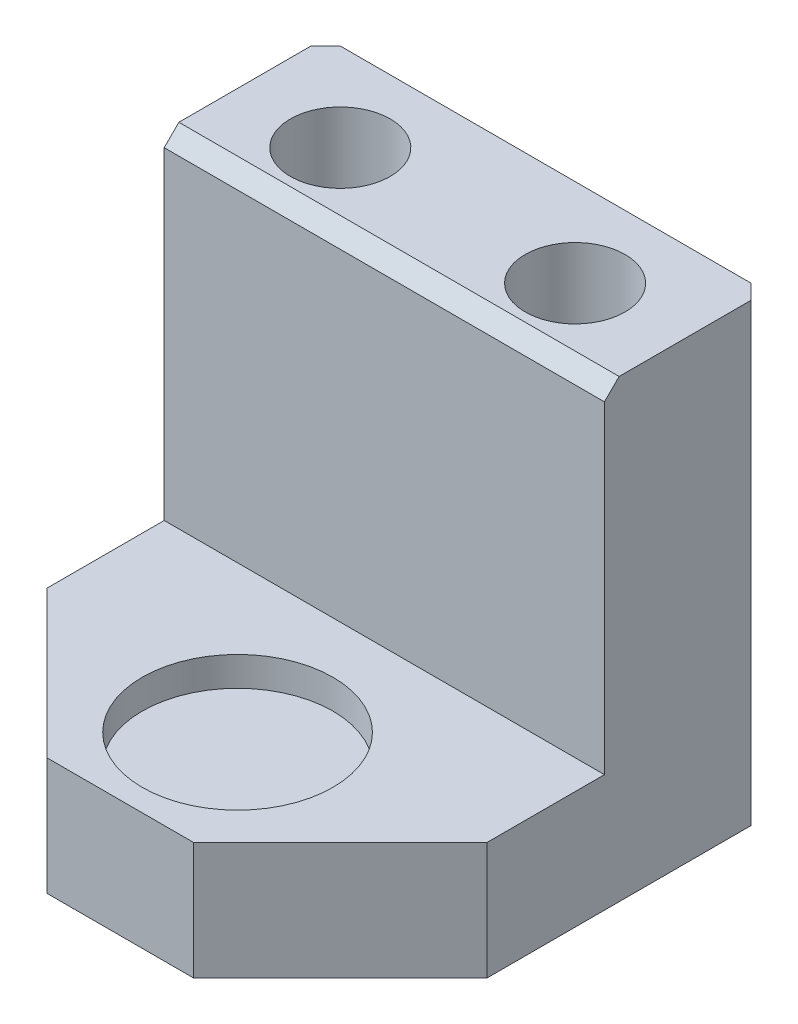
SolidWorks part; units mm, degrees
ref_plane "Front Plane" through (0, 0, 0) normal (0, 0, 1) x (1, 0, 0)
ref_plane "Top Plane" through (0, 0, 0) normal (0, 1, 0) x (1, 0, 0)
ref_plane "Right Plane" through (0, 0, 0) normal (1, 0, 0) x (0, 0, -1)
sketch "Sketch1" plane through (0, 0, 0) normal (0, 0, 1) x (1, 0, 0)
  line L1 (-7.5, -7.75) -> (7.5, -7.75)
  line L2 (-7.5, -7.75) -> (-7.5, 7.75)
  line L3 (-7.5, 7.75) -> (7.5, 7.75)
  line L4 (7.5, -7.75) -> (7.5, 7.75)
  line L5 (-7.5, -7.75) -> (7.5, 7.75) construction
  line L6 (-7.5, 7.75) -> (7.5, -7.75) construction
  point P0 (0, 0)
  dimension "D1" = 15
  dimension "D2" = 15.5
extrude "Boss-Extrude1" add sketch "Sketch1" along normal blind 6
sketch "Sketch2" plane through (0, 0, 6) normal (0, 0, 1) x (1, 0, 0)
  line L0 (7.5, -7.75) -> (7.5, 7.75) construction
  line L1 (-7.5, -7.75) -> (7.5, -7.75)
  line L2 (-7.5, -7.75) -> (-7.5, -3.75)
  line L3 (-7.5, -3.75) -> (7.5, -3.75)
  line L4 (7.5, -7.75) -> (7.5, -3.75)
  dimension "D1" = 4
extrude "Boss-Extrude2" add sketch "Sketch2" along normal blind 9
sketch "Sketch3" plane through (0, -3.75, 0) normal (0, 1, 0) x (1, 0, 0)
  line L0 (0, 0) -> (0, -20.2651) construction
  circle A0 centre (0, -11) radius 3.25
  dimension "D2" = 6.5
  dimension "D1" = 11
extrude "Cut-Extrude1" cut sketch "Sketch3" against normal blind 1
sketch "Sketch5" plane through (0, -3.75, 0) normal (0, 1, 0) x (1, 0, 0)
  circle A0 centre (0, -11) radius 2
  dimension "D1" = 4
extrude "Cut-Extrude2" [suppressed] cut sketch "Sketch5" against normal through all
hole_wizard "Hole size per socket head cap screw type 1" positions "Sketch7" profile "Sketch6" counterbore size "M3" standard "Gb" end condition through all
sketch "Sketch7" plane through (0, -7.75, 0) normal (0, -1, 0) x (-1, 0, 0)
  line L1 (4, -3.5) -> (-4, -3.5) construction
  line L3 (0, 0) -> (0, -6.7603) construction
  line L5 (7.5, 0) -> (-7.5, 0) construction
  point P0 (4, -3.5)
  point P9 (-4, -3.5)
  dimension "D1" = 8
  dimension "D2" = 3.5
sketch "Sketch6" plane through (-4, -7.75, 3.5) normal (1, 0, 0) x (0, 0, -1)
  line L0 (0, 0) -> (0, 15.5)
  line L1 (0, 15.5) -> (1.7, 15.5)
  line L3 (1.7, 15.5) -> (1.7, 3.4)
  line L4 (1.7, 3.4) -> (3, 3.4)
  line L5 (3, 3.4) -> (3, 0)
  line L7 (3, 0) -> (0, 0)
  line L11 (0, -6.35) -> (0, 107.95) construction
  dimension "通孔孔直径" = 3.4
  dimension "通孔孔深度" = 15.5
  dimension "柱形沉头孔直径" = 6
  dimension "柱形沉头孔深度" = 3.4
chamfer "Chamfer1" distance 5 angle 45 2 edges at (-7.5, -5.75, 15) (7.5, -5.75, 15)
chamfer "Chamfer2" distance 1 angle 45 2 edges at (7.5, 0, 0) (-7.5, 0, 0)
chamfer "Chamfer3" distance 0.5 angle 45 2 edges at (0, 7.75, 6) (0, 7.75, 0)
